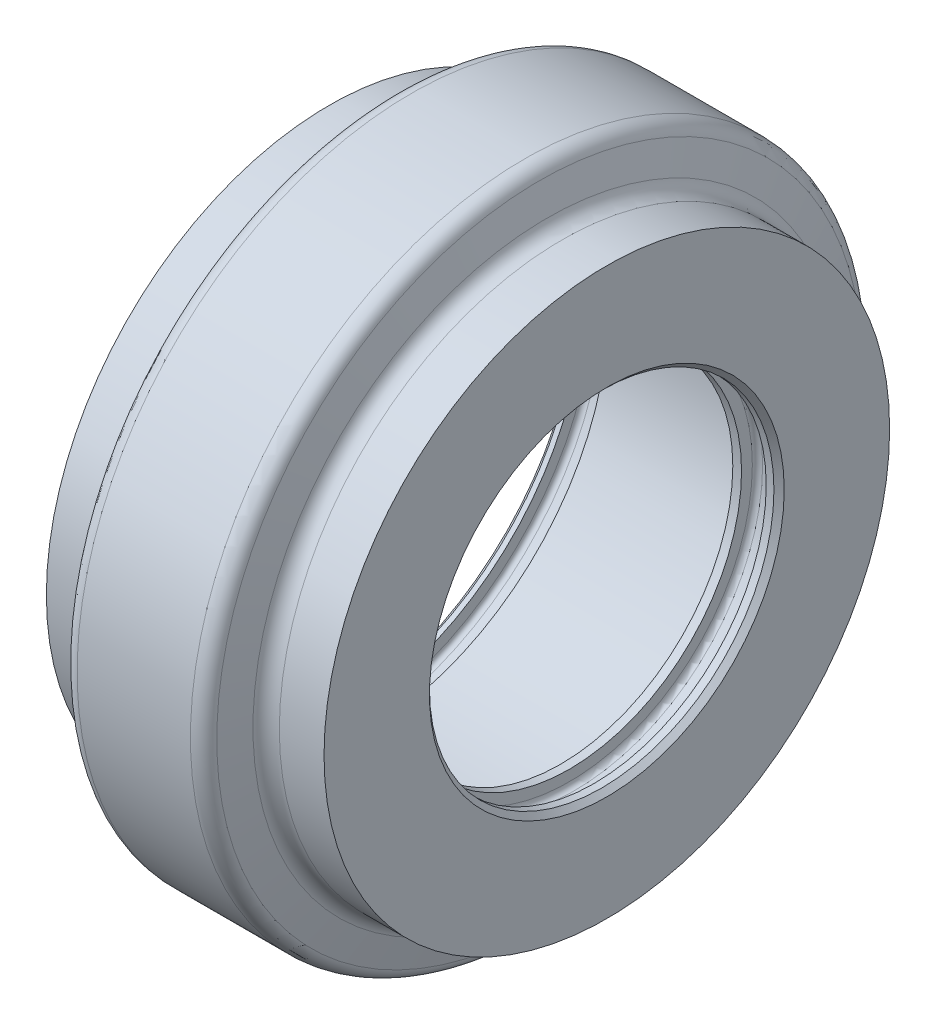
from build123d import *

# Parameters (mm, degrees)
CHAMFER1_SIZE = 1


with BuildPart() as part:
    # Sketch1 → Revolve1 (revolve)
    with BuildSketch(Plane.XY, mode=Mode.PRIVATE) as revolve1_sk:
        with BuildLine():
            Line((-27, 47.5), (-27, 55))
            Line((-27, 55), (-18.301980964, 55))
            ThreePointArc((-18.301980964, 55), (-16.475696677, 55.619939979), (-15.404203485, 57.223542865))
            Line((-15.404203485, 57.223542865), (-13.916304591, 62.776457135))
            ThreePointArc((-13.916304591, 62.776457135), (-12.844811399, 64.380060021), (-11.018527112, 65))
            Line((-11.018527112, 65), (11.018527112, 65))
            ThreePointArc((11.018527112, 65), (12.844811399, 64.380060021), (13.916304591, 62.776457135))
            Line((13.916304591, 62.776457135), (15.404203485, 57.223542865))
            ThreePointArc((15.404203485, 57.223542865), (16.475696677, 55.619939979), (18.301980964, 55))
            Line((18.301980964, 55), (27, 55))
            Line((27, 55), (27, 33.5))
            Line((27, 33.5), (24.5, 33.5))
            Line((24.5, 33.5), (24.5, 35.6))
            ThreePointArc((24.5, 35.6), (24.207106781, 36.307106781), (23.5, 36.6))
            Line((23.5, 36.6), (20.7, 36.6))
            ThreePointArc((20.7, 36.6), (19.992893219, 36.307106781), (19.7, 35.6))
            Line((19.7, 35.6), (19.7, 33.5))
            Line((19.7, 33.5), (18, 33.5))
            Line((18, 33.5), (18, 47.5))
            Line((18, 47.5), (-20.2, 47.5))
            Line((-20.2, 47.5), (-20.2, 49.6))
            ThreePointArc((-20.2, 49.6), (-20.492893219, 50.307106781), (-21.2, 50.6))
            Line((-21.2, 50.6), (-24, 50.6))
            ThreePointArc((-24, 50.6), (-24.707106781, 50.307106781), (-25, 49.6))
            Line((-25, 49.6), (-25, 47.5))
            Line((-25, 47.5), (-27, 47.5))
        make_face()
    revolve(revolve1_sk.sketch.rotate(Axis((27, 0, 0), (-1, 0, 0)), 90), axis=Axis((27, 0, 0), (-1, 0, 0)))

    # Chamfer1
    chamfer1_edges = [part.edges().sort_by_distance(p)[0] for p in [
        (-27, 0, 47.5),
        (27, 0, 33.5),
    ]]
    chamfer(chamfer1_edges, length=CHAMFER1_SIZE)


solid = part.part
